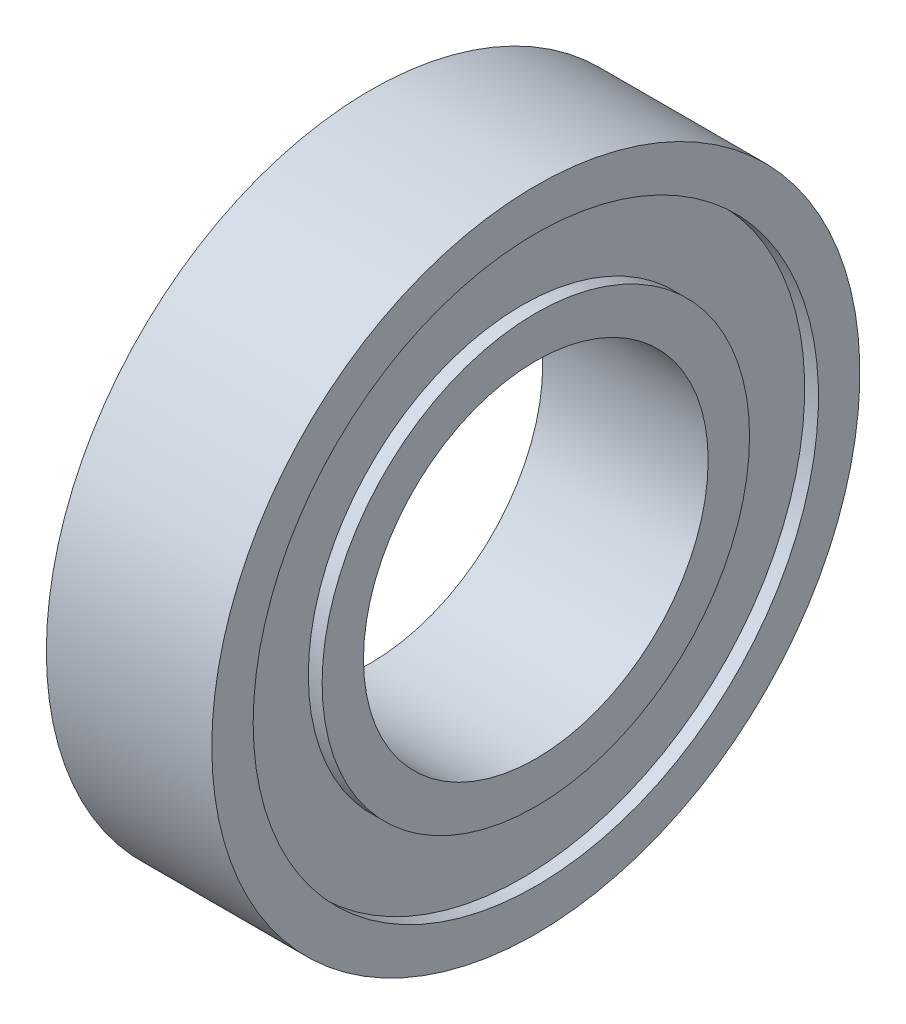
SolidWorks part; units mm, degrees
ref_plane "Front Plane" through (0, 0, 0) normal (0, 0, 1) x (1, 0, 0)
ref_plane "Top Plane" through (0, 0, 0) normal (0, 1, 0) x (1, 0, 0)
ref_plane "Right Plane" through (0, 0, 0) normal (1, 0, 0) x (0, 0, -1)
sketch "Sketch1" plane through (0, 0, 0) normal (0, 0, 1) x (1, 0, 0)
  line L0 (0, 0) -> (47.5348, 0) construction
  line L1 (13.1202, 20.5) -> (13.1202, 23.5)
  line L2 (13.1202, 12.5) -> (25.1202, 12.5)
  line L3 (13.1202, 12.5) -> (13.1202, 15.5)
  line L4 (13.1202, 23.5) -> (25.1202, 23.5)
  line L5 (25.1202, 12.5) -> (25.1202, 15.5)
  line L6 (13.1202, 15.5) -> (14.1202, 15.5)
  line L7 (25.1202, 20.5) -> (25.1202, 23.5)
  line L8 (13.1202, 20.5) -> (14.1202, 20.5)
  line L9 (14.1202, 15.5) -> (14.1202, 20.5)
  line L10 (25.1202, 15.5) -> (24.1202, 15.5)
  line L12 (25.1202, 20.5) -> (24.1202, 20.5)
  line L13 (24.1202, 15.5) -> (24.1202, 20.5)
  dimension "D1" = 12
  dimension "D2" = 25
  dimension "D3" = 47
  dimension "D4" = 1
  dimension "D5" = 3
revolve "Revolve1" add sketch "Sketch1" angle 360 about L0
